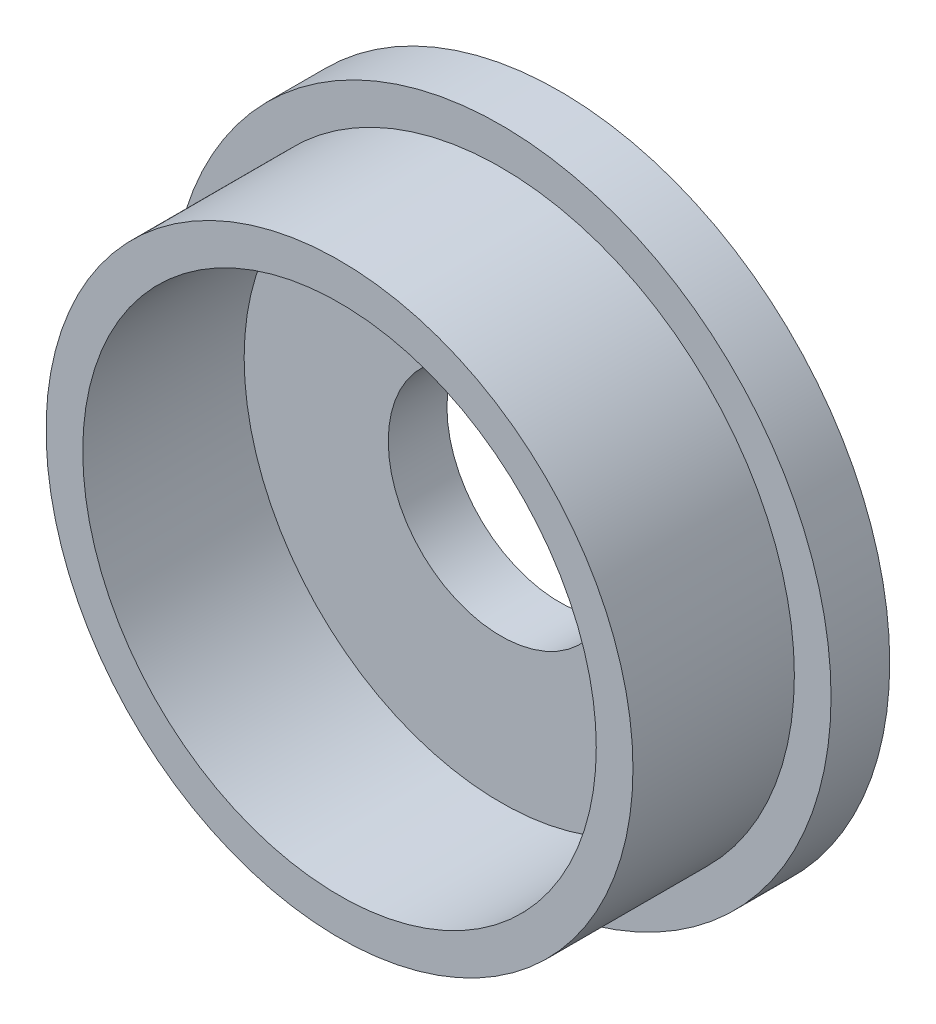
from build123d import *

# Parameters (mm, degrees)
SKETCH_1_R          = 22.5
EXTRUDE_1_DEPTH     = 2
SKETCH_2_R          = 20
SKETCH_2_R_2        = 17.5
EXTRUDE_2_DEPTH     = 11
SKETCH_3_R          = 7.678665591
CUT_EXTRUDE_1_DEPTH = 21


with BuildPart() as part:
    # 草图1 → 凸台-拉伸1 (new, symmetric)
    with BuildSketch(Plane.XY):
        Circle(SKETCH_1_R)
    extrude(amount=EXTRUDE_1_DEPTH, both=True)

    # 草图2 → 凸台-拉伸2 (add)
    with BuildSketch(Plane.XY.offset(2)):
        Circle(SKETCH_2_R)
        Circle(SKETCH_2_R_2, mode=Mode.SUBTRACT)
    extrude(amount=EXTRUDE_2_DEPTH)

    # 草图3 → 切除-拉伸1 (cut)
    with BuildSketch(Plane.XY.offset(2)):
        Circle(SKETCH_3_R)
    extrude(amount=-CUT_EXTRUDE_1_DEPTH, mode=Mode.SUBTRACT)


solid = part.part
